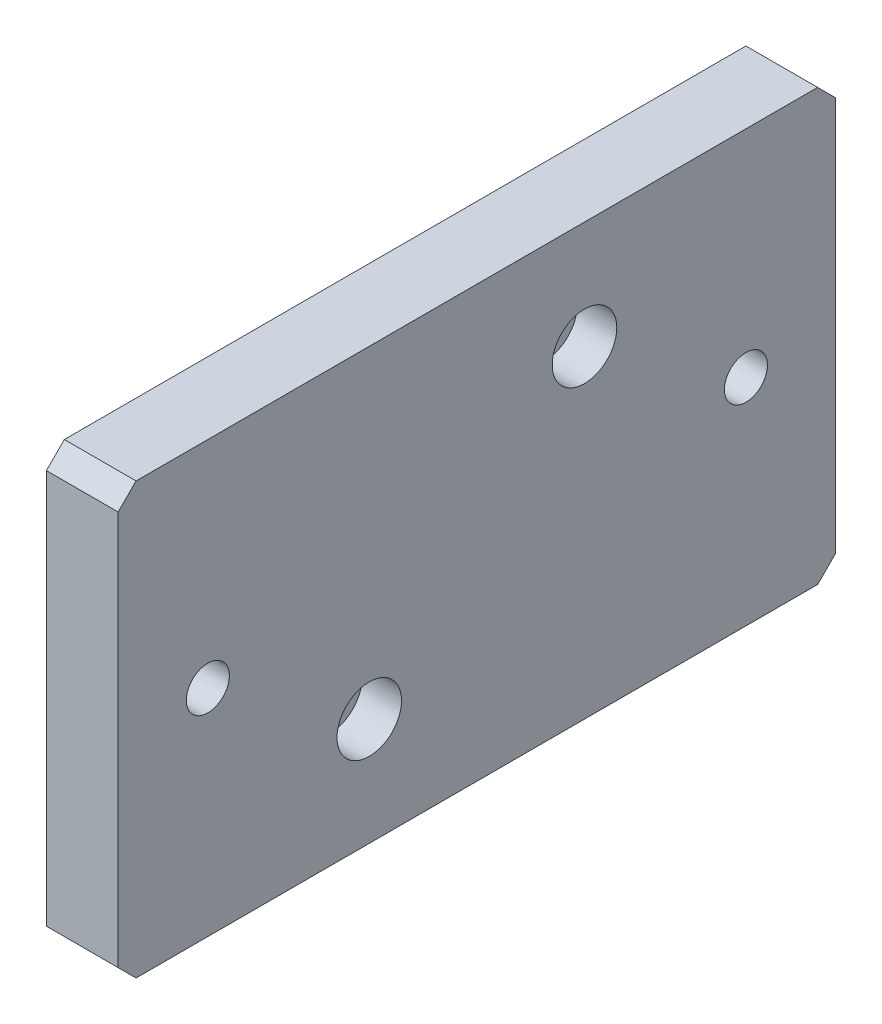
from build123d import *

# Parameters (mm, degrees)
SKETCH_1_W                = 200
SKETCH_1_H                = 120
EXTRUDE_1_DEPTH           = 20
HOLE_WIZARD_1_D           = 11
HOLE_WIZARD_1_CBORE_D     = 18
HOLE_WIZARD_1_CBORE_DEPTH = 11
HOLE_WIZARD_M14_1_D       = 12
CHAMFER_1_SIZE            = 5


with BuildPart() as part:
    # 草图1 → 凸台-拉伸1 (new body)
    with BuildSketch(Plane(origin=(0, 0, 0), x_dir=(0, 0, -1), z_dir=(1, 0, 0))):
        Rectangle(SKETCH_1_W, SKETCH_1_H)
    extrude(amount=EXTRUDE_1_DEPTH)

    # 打孔尺寸(%根据)内六角圆柱头螺钉的类型1 (through all)
    with Locations(Plane(origin=(20, 0, 0), x_dir=(0, 0, -1), z_dir=(1, 0, 0))):
        with Locations((30, 30), (-30, -30)):
            CounterBoreHole(HOLE_WIZARD_1_D / 2, HOLE_WIZARD_1_CBORE_D / 2, HOLE_WIZARD_1_CBORE_DEPTH)

    # M14 螺纹孔1 (through all)
    with Locations(Plane(origin=(20, 0, 0), x_dir=(0, 0, -1), z_dir=(1, 0, 0))):
        with Locations((-75, 0), (75, 0)):
            Hole(HOLE_WIZARD_M14_1_D / 2)

    # 倒角1
    chamfer_1_edges = [part.edges().sort_by_distance(p)[0] for p in [
        (10, -60, -100),
        (10, -60, 100),
        (10, 60, 100),
        (10, 60, -100),
    ]]
    chamfer(chamfer_1_edges, length=CHAMFER_1_SIZE)


solid = part.part
